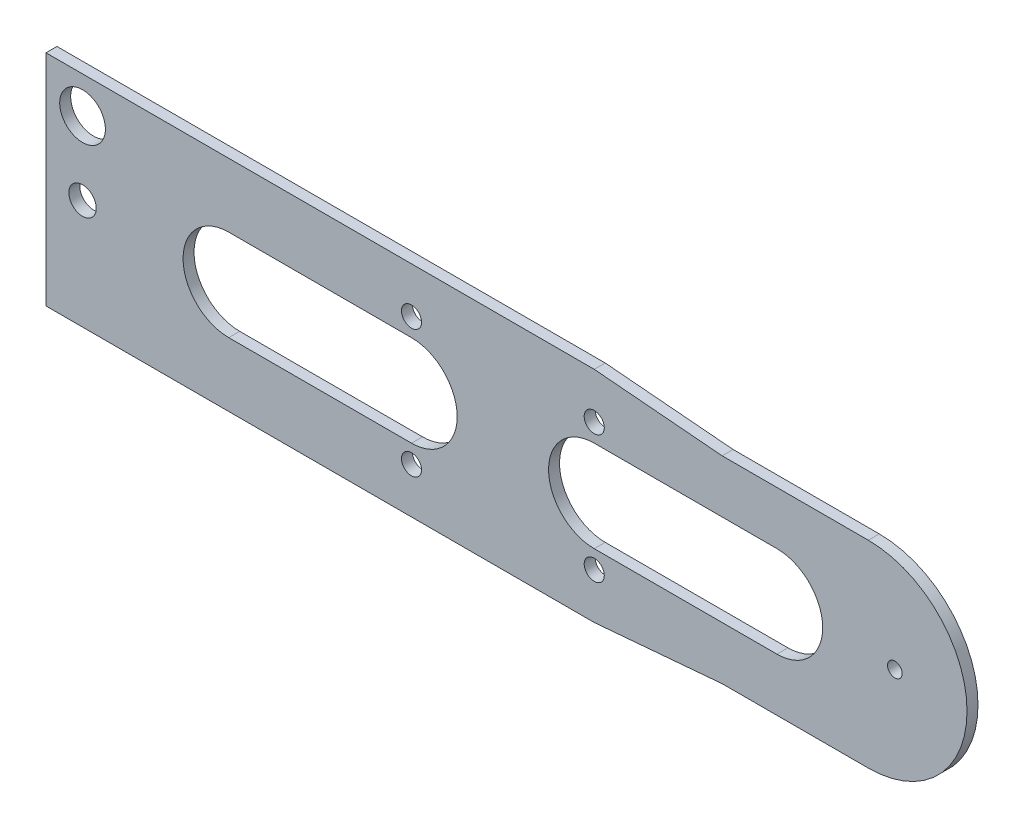
SolidWorks part; units mm, degrees
material "Zoltek Panex 33"
ref_plane "前视基准面" through (0, 0, 0) normal (0, 0, 1) x (1, 0, 0)
ref_plane "上视基准面" through (0, 0, 0) normal (0, 1, 0) x (1, 0, 0)
ref_plane "右视基准面" through (0, 0, 0) normal (1, 0, 0) x (0, 0, -1)
other "Configuration Table"
sketch "草图1" plane through (0, 0, 0) normal (0, 0, 1) x (1, 0, 0)
  line L0 (-255, 0) -> (45, 0)
  line L1 (-255, 0) -> (-255, 120)
  line L2 (-235, 120) -> (45, 120)
  line L9 (45, 120) -> (115, 114)
  line L10 (45, 0) -> (115, 6)
  line L13 (-255, 120) -> (-235, 120)
  line L14 (115, 114) -> (195, 114)
  line L15 (115, 6) -> (195, 6)
  line L16 (-155, 60) -> (-55, 60) construction
  line L17 (-155, 85) -> (-55, 85)
  line L18 (-155, 35) -> (-55, 35)
  line L20 (45, 60) -> (145, 60) construction
  line L21 (45, 85) -> (145, 85)
  line L22 (45, 35) -> (145, 35)
  arc A1 (-155, 85) -> (-155, 35) centre (-155, 60) ccw
  arc A2 (-55, 35) -> (-55, 85) centre (-55, 60) ccw
  arc A3 (45, 85) -> (45, 35) centre (45, 60) ccw
  arc A4 (145, 35) -> (145, 85) centre (145, 60) ccw
  circle A5 centre (-235, 100) radius 12.5
  circle A6 centre (-235, 60) radius 7.5
  arc A10 (195, 6) -> (195, 114) centre (195, 60) ccw
  point P4 (0, 0)
  point P11 (-255, 60)
  point P16 (-105, 60)
  point P26 (95, 60)
  point P33 (-105, 60)
  dimension "D5" = 25
  dimension "D10" = 15
  dimension "D2" = 120
  dimension "D3" = 300
  dimension "D4" = 20
  dimension "D6" = 100
  dimension "D7" = 50
  dimension "D8" = 100
  dimension "D9" = 50
  dimension "D11" = 80
  dimension "D12" = 80
extrude "凸台-拉伸1" add sketch "草图1" along normal blind 6
sketch "草图4" plane through (0, 0, 0) normal (0, 0, 1) x (1, 0, 0)
  line L0 (-55, 85) -> (-55, 95) construction
  line L1 (-55, 35) -> (-55, 25)
  line L2 (45, 85) -> (45, 95)
  line L3 (45, 35) -> (45, 25)
  dimension "D1" = 10
  dimension "D2" = 10
hole_wizard "M6 六角圆柱头螺钉的柱形沉头孔1" positions "草图5" profile "草图6" counterbore size "M6" standard "GB" end condition through all
sketch "草图5" plane through (0, 0, 6) normal (0, 0, 1) x (1, 0, 0)
  point P0 (-55, 95)
  point P3 (-55, 25)
  point P6 (45, 95)
  point P9 (45, 25)
sketch "草图6" plane through (-55, 95, 6) normal (1, 0, 0) x (0, -1, 0)
  line L0 (0, 0) -> (0, 6)
  line L1 (0, 6) -> (3.5, 6)
  line L3 (3.5, 6) -> (3.5, 6.8)
  line L4 (3.5, 6.8) -> (5.5, 6.8)
  line L5 (5.5, 6.8) -> (5.5, 0)
  line L7 (5.5, 0) -> (0, 0)
  line L11 (0, -6.35) -> (0, 107.95) construction
  dimension "通孔孔直径" = 7
  dimension "通孔孔深度" = 6
  dimension "柱形沉头孔直径" = 11
  dimension "柱形沉头孔深度" = 6.8
sketch "草图7" plane through (0, 0, 0) normal (0, 0, -1) x (-1, 0, 0)
  circle A2 centre (-209.5, 60) radius 4
  dimension "D1" = 8
extrude "切除-拉伸1" cut sketch "草图7" against normal blind 10
